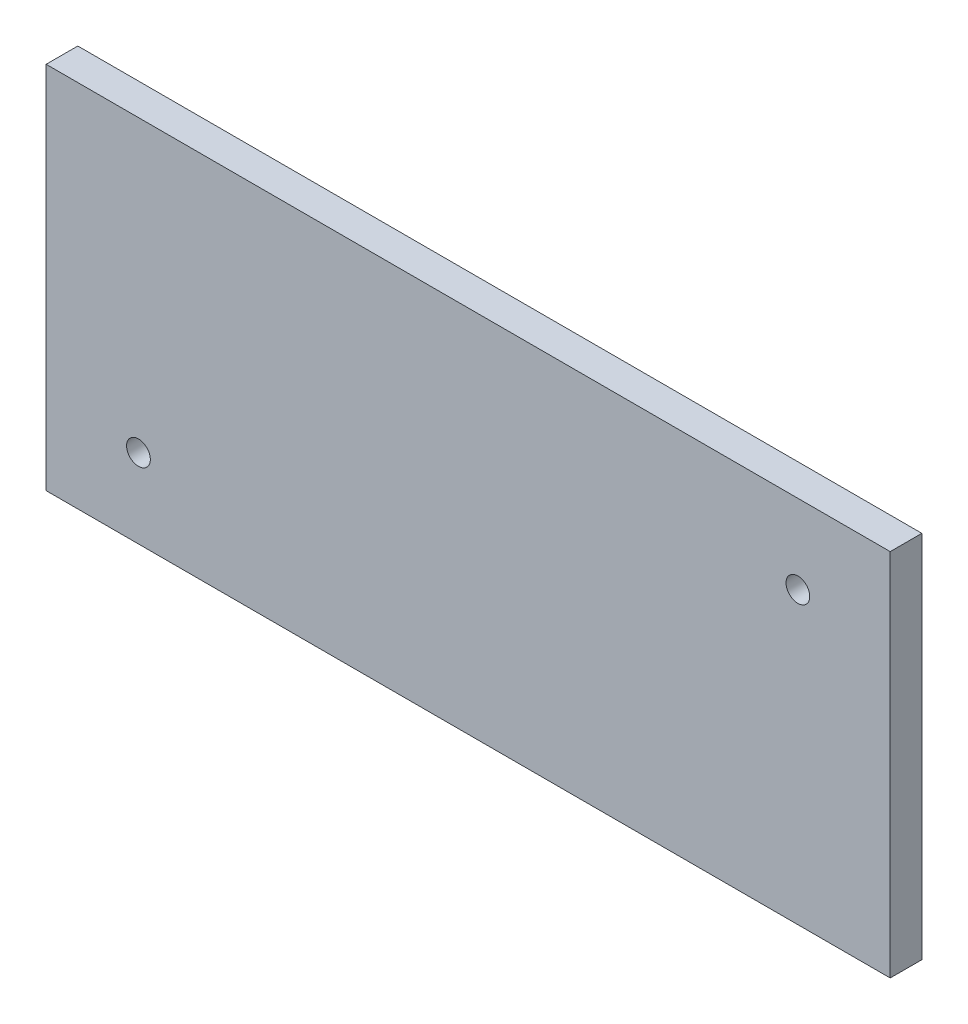
from build123d import *

# Parameters (mm, degrees)
SKETCH_1_W          = 320
SKETCH_1_H          = 140
EXTRUDE_1_DEPTH     = 6
SKETCH_2_R          = 4.5
CUT_EXTRUDE_1_DEPTH = 16


with BuildPart() as part:
    # 草图1 → 凸台-拉伸1 (new, symmetric)
    with BuildSketch(Plane.XY):
        Rectangle(SKETCH_1_W, SKETCH_1_H)
    extrude(amount=EXTRUDE_1_DEPTH, both=True)

    # 草图2 → 切除-拉伸1 (cut, symmetric)
    with BuildSketch(Plane.XY):
        with Locations((-125, -40)):
            Circle(SKETCH_2_R)
        with Locations((125, 40)):
            Circle(SKETCH_2_R)
    extrude(amount=CUT_EXTRUDE_1_DEPTH, both=True, mode=Mode.SUBTRACT)


solid = part.part
